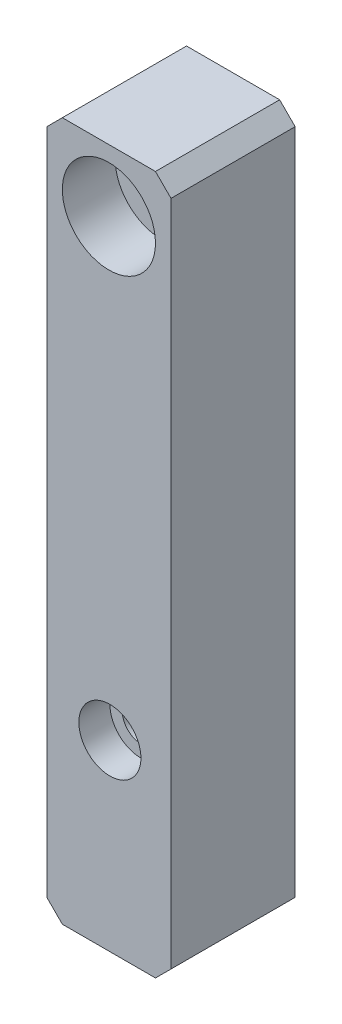
SolidWorks part; units mm, degrees
ref_plane "Front Plane" through (0, 0, 0) normal (0, 0, 1) x (1, 0, 0)
ref_plane "Top Plane" through (0, 0, 0) normal (0, 1, 0) x (1, 0, 0)
ref_plane "Right Plane" through (0, 0, 0) normal (1, 0, 0) x (0, 0, -1)
sketch "Sketch1" plane through (0, 0, 0) normal (0, 0, 1) x (1, 0, 0)
  line L1 (-14.3445, -5) -> (-6.3445, -5)
  line L2 (-14.3445, -5) -> (-14.3445, -50)
  line L3 (-14.3445, -50) -> (-6.3445, -50)
  line L4 (-6.3445, -5) -> (-6.3445, -50)
  dimension "D1" = 8
  dimension "D2" = 45
extrude "Boss-Extrude1" add sketch "Sketch1" along normal blind 8 contours L4 L3 L2 L1
sketch "Sketch2" plane through (0, 0, 8) normal (0, 0, 1) x (1, 0, 0)
  line L0 (-21.5533, -9) -> (-3.3922, -9) construction
  line L1 (-10.3445, -50) -> (-10.3445, 0) construction
  line L2 (-14.3445, -50) -> (-6.3445, -50) construction
  line L3 (-14.3445, -5) -> (-6.3445, -5) construction
  circle A0 centre (-10.2812, -38.2) radius 2
  dimension "D2" = 4
  dimension "D1" = 4
hole_wizard "Hole size (per socket head cap screw type)1" positions "3DSketch2" profile "Sketch3" counterbore size "M3" standard "GB" end condition through all
sketch3d "3DSketch2"
  line L0 (-21.5533, -9, 8) -> (-3.3922, -9, 8) construction
  line L1 (-10.3445, -50, 8) -> (-10.3445, 0, 8) construction
  point P0 (-10.3445, -9, 8)
sketch "Sketch3" plane through (-10.3445, -9, 8) normal (1, 0, 0) x (0, -1, 0)
  line L0 (0, 0) -> (0, 8)
  line L1 (0, 8) -> (1.7, 8)
  line L3 (1.7, 8) -> (1.7, 3.4)
  line L4 (1.7, 3.4) -> (3, 3.4)
  line L5 (3, 3.4) -> (3, 0)
  line L7 (3, 0) -> (0, 0)
  line L11 (0, -6.35) -> (0, 107.95) construction
  dimension "通孔孔直径" = 3.4
  dimension "通孔孔深度" = 8
  dimension "柱形沉头孔直径" = 6
  dimension "柱形沉头孔深度" = 3.4
extrude "Cut-Extrude1" cut sketch "Sketch2" against normal blind 2 contours A0
sketch "Sketch4" plane through (0, 0, 0) normal (0, 0, -1) x (-1, 0, 0)
  line L0 (10.3445, -2.2669) -> (10.3445, -58.8455) construction
  line L1 (10.2812, -38.2) -> (20.1799, -38.2) construction
hole_wizard "Hole size (per socket head cap screw type)2" positions "3DSketch3" profile "Sketch5" counterbore size "M2" standard "GB" end condition through all
sketch3d "3DSketch3"
  point P0 (-10.2812, -38.2, 0)
sketch "Sketch5" plane through (-10.2812, -38.2, 0) normal (1, 0, 0) x (0, 1, 0)
  line L0 (0, 0) -> (0, 8)
  line L1 (0, 8) -> (1.2, 8)
  line L3 (1.2, 8) -> (1.2, 2.3)
  line L4 (1.2, 2.3) -> (2.15, 2.3)
  line L5 (2.15, 2.3) -> (2.15, 0)
  line L7 (2.15, 0) -> (0, 0)
  line L11 (0, -6.35) -> (0, 107.95) construction
  dimension "通孔孔直径" = 2.4
  dimension "通孔孔深度" = 8
  dimension "柱形沉头孔直径" = 4.3
  dimension "柱形沉头孔深度" = 2.3
chamfer "Chamfer1" distance 1 angle 45 4 edges at (-6.3445, -50, 4) (-14.3445, -50, 4) (-6.3445, -5, 4) (-14.3445, -5, 4)
